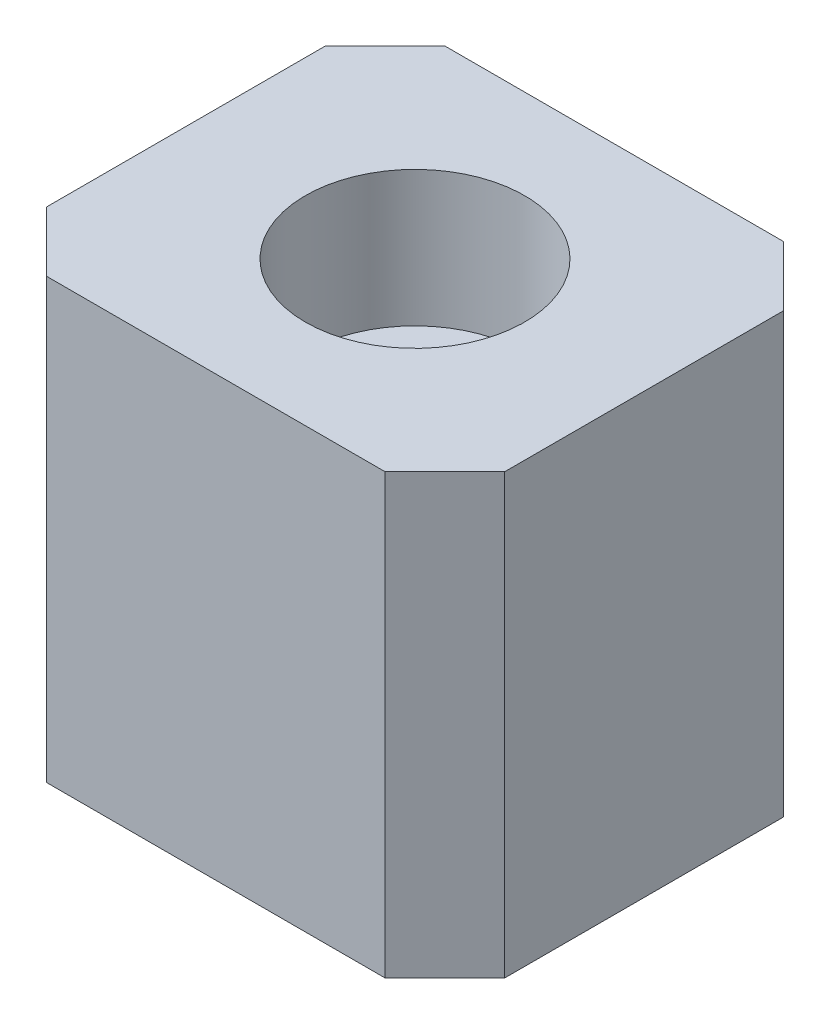
from build123d import *

# Parameters (mm, degrees)
SKETCH_1_W                = 23
SKETCH_1_H                = 22
EXTRUDE_1_DEPTH           = 20
HOLE_WIZARD_1_D           = 6.6
HOLE_WIZARD_1_CBORE_D     = 11
HOLE_WIZARD_1_CBORE_DEPTH = 6.8
CHAMFER_1_SIZE            = 3


with BuildPart() as part:
    # 草图1 → 凸台-拉伸1 (new body)
    with BuildSketch(Plane.XY):
        with Locations((0, 11)):
            Rectangle(SKETCH_1_W, SKETCH_1_H)
    extrude(amount=EXTRUDE_1_DEPTH)

    # 打孔尺寸(%根据)内六角圆柱头螺钉的类型1 (through all)
    with Locations(Plane(origin=(0, 22, 0), x_dir=(1, 0, 0), z_dir=(0, 1, 0))):
        with Locations((0, -10)):
            CounterBoreHole(HOLE_WIZARD_1_D / 2, HOLE_WIZARD_1_CBORE_D / 2, HOLE_WIZARD_1_CBORE_DEPTH)

    # 倒角1
    chamfer_1_edges = [part.edges().sort_by_distance(p)[0] for p in [
        (11.5, 11, 20),
        (-11.5, 11, 20),
        (11.5, 11, 0),
        (-11.5, 11, 0),
    ]]
    chamfer(chamfer_1_edges, length=CHAMFER_1_SIZE)


solid = part.part
